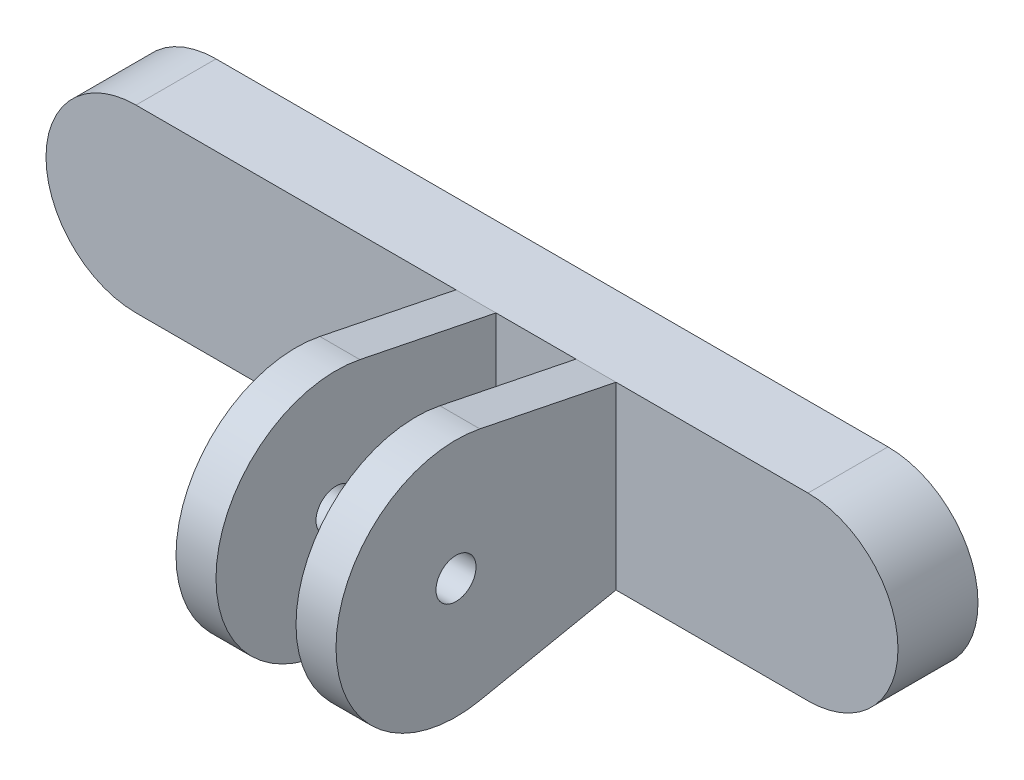
from build123d import *

# Parameters (mm, degrees)
BOSS_EXTRUDE_1_DEPTH     = 2
SKETCH_3_R               = 0.5
BOSS_EXTRUDE_2_DEPTH     = 4
CUT_EXTRUDE_1_DEPTH      = 22.281643835
CUT_EXTRUDE_1_DEPTH_BACK = 22.281643835
SKETCH_4_W               = 2
SKETCH_4_H               = 8.093157612


with BuildPart() as part:
    # Sketch 1 → Boss-Extrude 1 (new body)
    with BuildSketch(Plane.XY):
        with BuildLine():
            Line((0, 2.25), (16.8, 2.25))
            ThreePointArc((16.8, 2.25), (19.05, 0), (16.8, -2.25))
            Line((16.8, -2.25), (0, -2.25))
            ThreePointArc((0, -2.25), (-2.25, 0), (0, 2.25))
        make_face()
    extrude(amount=BOSS_EXTRUDE_1_DEPTH)

    # Sketch 3 → Boss-Extrude 2 (add)
    with BuildSketch(Plane.ZY.offset(-12)):
        with BuildLine():
            Line((2, 2.25), (2, -2.249022682))
            Line((2, -2.249022682), (5.403845626, -2.939192745))
            ThreePointArc((5.403845626, -2.939192745), (8.999999942, 0.001391019), (5.403034747, 2.940982849))
            Line((5.403034747, 2.940982849), (2, 2.25))
        make_face()
        with Locations((5.99999997, 0.000977318)):
            Circle(SKETCH_3_R, mode=Mode.SUBTRACT)
    extrude(amount=BOSS_EXTRUDE_2_DEPTH)

    # Sketch 4 → Cut-Extrude 1 (cut, two sides: drawn at the far end of the back side and taken through both)
    with BuildSketch(Plane(origin=(0, 0, 0), x_dir=(1, 0, 0), z_dir=(0, 1, 0)).offset(-CUT_EXTRUDE_1_DEPTH_BACK)):
        with Locations((10, -6.046578806)):
            Rectangle(SKETCH_4_W, SKETCH_4_H)
    extrude(amount=CUT_EXTRUDE_1_DEPTH + CUT_EXTRUDE_1_DEPTH_BACK, mode=Mode.SUBTRACT)


solid = part.part
